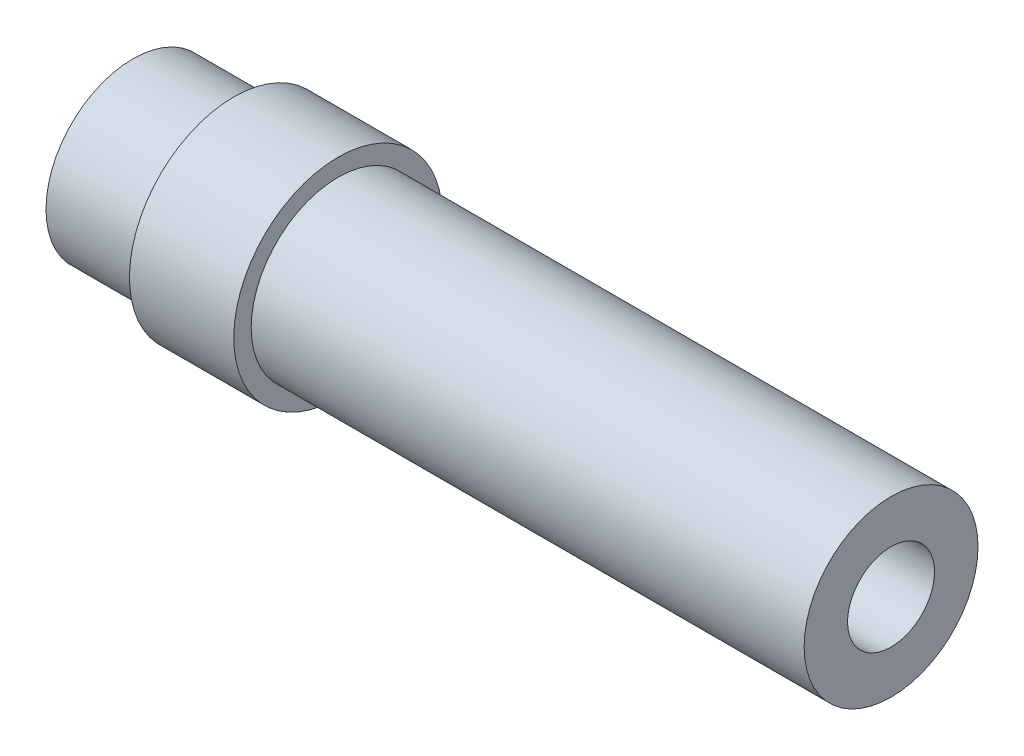
SolidWorks part; units mm, degrees
ref_plane "Front" through (0, 0, 0) normal (0, 0, 1) x (1, 0, 0)
ref_plane "Top" through (0, 0, 0) normal (0, 1, 0) x (1, 0, 0)
ref_plane "Right" through (0, 0, 0) normal (1, 0, 0) x (0, 0, -1)
sketch "Sketch1" plane through (0, 0, 0) normal (0, 0, 1) x (1, 0, 0)
  line L0 (22.3057, -2.5) -> (0.5057, -2.5)
  line L1 (3.4057, 0) -> (3.4057, 0.5)
  line L2 (3.4057, 0.5) -> (6.4057, 0.5)
  line L3 (6.4057, 0.5) -> (6.4057, 0)
  line L4 (6.4057, 0) -> (22.3057, 0)
  line L5 (22.3057, 0) -> (22.3057, -2.5)
  line L6 (0.5057, -2.5) -> (0.5057, 0)
  line L7 (0.5057, 0) -> (3.4057, 0)
  dimension "D1" = 3
  dimension "D2" = 21.8
  dimension "D3" = 2.9
  dimension "D4" = 0.5
  dimension "D5" = 2.5
  dimension "D6" = 2.5
revolve "Revolve1" add sketch "Sketch1" angle 360 about L0
hole_wizard "M3 Tapped Hole1" positions "3DSketch1" profile "Sketch3" tap size "M3" standard "GB"
sketch3d "3DSketch1"
  line L0 (0.5057, -2.5, 0) -> (3.4057, -2.5, 0) construction
  line L1 (6.4057, -2.5, 0) -> (22.3057, -2.5, 0) construction
  point P0 (0.5057, -2.5, 0)
  point P4 (22.3057, -2.5, 0)
sketch "Sketch3" plane through (0.5057, -2.5, 0) normal (0, 1, 0) x (0, 0, 1)
  line L0 (0, 0) -> (0, 8.7511)
  line L1 (0, 8.7511) -> (1.25, 8)
  line L2 (1.25, 8) -> (1.25, 0)
  line L5 (1.25, 0) -> (0, 0)
  line L10 (0, 8.7511) -> (-1.25, 8) construction
  line L11 (0, -6.35) -> (0, 107.95) construction
  dimension "螺纹孔钻头直径" = 2.5
  dimension "螺纹孔钻头深度" = 8
  dimension "导头角度" = 118
cosmetic thread "CosmeticThread1"
cosmetic thread "CosmeticThread2"
